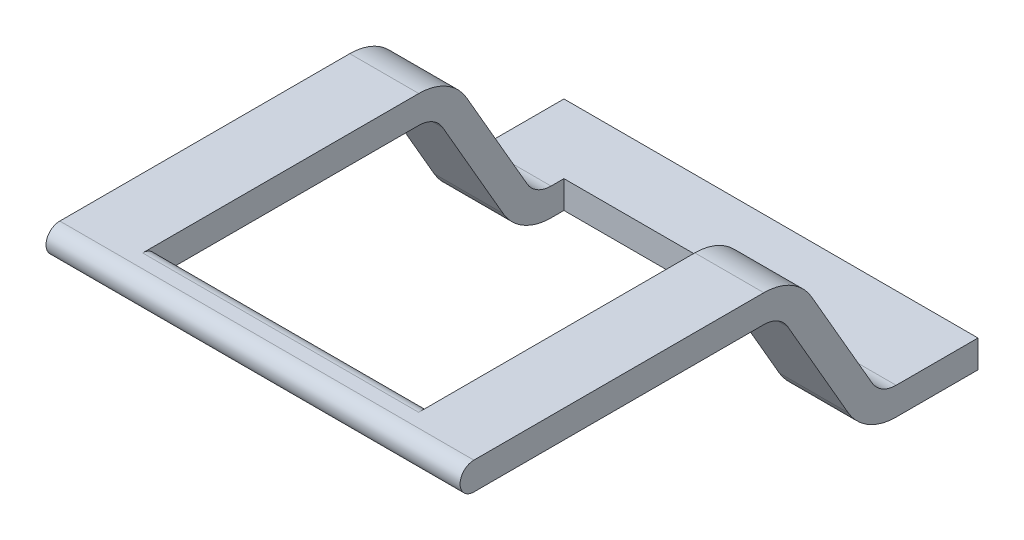
from build123d import *

# Parameters (mm, degrees)
BOSS_EXTRUDE1_DEPTH = 30
CUT_EXTRUDE1_START  = -5
CUT_EXTRUDE1_DEPTH  = 5
BOSS_EXTRUDE2_DEPTH = 1
SKETCH4_W           = 5
SKETCH4_H           = 2
BOSS_EXTRUDE3_DEPTH = 20.16339138
SKETCH5_W           = 5
SKETCH5_H           = 10.599022434
BOSS_EXTRUDE4_DEPTH = 1.154700538
CUT_EXTRUDE2_DEPTH  = 5
BOSS_EXTRUDE5_DEPTH = 1
SKETCH8_W           = 5
SKETCH8_H           = 2
BOSS_EXTRUDE6_DEPTH = 20.16339138
SKETCH9_W           = 5
SKETCH9_H           = 10.599022434
BOSS_EXTRUDE7_DEPTH = 1.154700538
BOSS_EXTRUDE8_DEPTH = 2
DRAFT1_ANGLE        = 30
DRAFT2_ANGLE        = 30
FILLET1_R           = 2
FILLET2_R           = 4


with BuildPart() as part:
    # Sketch1 → Boss-Extrude1 (new body)
    with BuildSketch(Plane(origin=(-30, 0, 0), x_dir=(0, -1, 0), z_dir=(-1, 0, 0))):
        with BuildLine():
            Line((0, -1), (0, -2))
            ThreePointArc((0, -2), (1, -3), (2, -2))
            Line((2, -2), (2, -1))
            ThreePointArc((2, -1), (1, 0), (0, -1))
        make_face()
    extrude(amount=-BOSS_EXTRUDE1_DEPTH)

    # Sketch2 → Cut-Extrude1 (cut)
    with BuildSketch(Plane(origin=(0, 0, 0), x_dir=(0, 0, -1), z_dir=(1, 0, 0)).offset(CUT_EXTRUDE1_START)):
        with BuildLine():
            Line((2, 0), (2, -2))
            ThreePointArc((2, -2), (3, -1), (2, 0))
        make_face()
    extrude(amount=CUT_EXTRUDE1_DEPTH, mode=Mode.SUBTRACT)

    # Sketch3 → Boss-Extrude2 (add)
    with BuildSketch(Plane(origin=(0, 0, -2), x_dir=(-1, 0, 0), z_dir=(0, 0, -1))):
        Polygon((5, -2), (0, -2), (0, 0), (5, 0), (5, -1), align=None)
    extrude(amount=BOSS_EXTRUDE2_DEPTH)

    # Sketch4 → Boss-Extrude3 (add)
    with BuildSketch(Plane(origin=(0, 0, -3), x_dir=(-1, 0, 0), z_dir=(0, 0, -1))):
        with Locations((2.5, -1)):
            Rectangle(SKETCH4_W, SKETCH4_H)
    extrude(amount=BOSS_EXTRUDE3_DEPTH)

    # Sketch5 → Boss-Extrude4 (add)
    with BuildSketch(Plane(origin=(0, 0, -23.16339138), x_dir=(-1, 0, 0), z_dir=(0, 0, -1))):
        with Locations((2.5, -5.299511217)):
            Rectangle(SKETCH5_W, SKETCH5_H)
    extrude(amount=BOSS_EXTRUDE4_DEPTH)

    # Sketch6 → Cut-Extrude2 (cut)
    with BuildSketch(Plane.ZY.offset(30)):
        with BuildLine():
            Line((-2, -2), (-2, 0))
            ThreePointArc((-2, 0), (-3, -1), (-2, -2))
        make_face()
    extrude(amount=-CUT_EXTRUDE2_DEPTH, mode=Mode.SUBTRACT)

    # Sketch7 → Boss-Extrude5 (add)
    with BuildSketch(Plane(origin=(0, 0, -2), x_dir=(-1, 0, 0), z_dir=(0, 0, -1))):
        Polygon((30, -2), (25, -2), (25, -1), (25, 0), (30, 0), align=None)
    extrude(amount=BOSS_EXTRUDE5_DEPTH)

    # Sketch8 → Boss-Extrude6 (add)
    with BuildSketch(Plane(origin=(0, 0, -3), x_dir=(-1, 0, 0), z_dir=(0, 0, -1))):
        with Locations((27.5, -1)):
            Rectangle(SKETCH8_W, SKETCH8_H)
    extrude(amount=BOSS_EXTRUDE6_DEPTH)

    # Sketch9 → Boss-Extrude7 (add)
    with BuildSketch(Plane(origin=(0, 0, -23.16339138), x_dir=(-1, 0, 0), z_dir=(0, 0, -1))):
        with Locations((27.5, -5.299511217)):
            Rectangle(SKETCH9_W, SKETCH9_H)
    extrude(amount=BOSS_EXTRUDE7_DEPTH)

    # Sketch10 → Boss-Extrude8 (add)
    with BuildSketch(Plane.XZ.offset(10.599022434)):
        Polygon((0, -23.16339138), (0, -37.525669468), (-30, -37.525669468), (-30, -23.16339138), (-25, -23.16339138), (-25, -32.525669468), (-5, -32.525669468), (-5, -23.16339138), align=None)
    extrude(amount=BOSS_EXTRUDE8_DEPTH)

    # Draft1
    draft1_faces = [part.faces().sort_by_distance(p)[0] for p in [
        (-2.5, -5.299511217, -24.318091918),
        (-27.5, -5.299511217, -24.318091918),
    ]]
    draft(draft1_faces, Plane(origin=(0, 0, -1), x_dir=(0, 0, 1), z_dir=(0, 1, 0)), DRAFT1_ANGLE)

    # Draft2
    draft2_faces = [part.faces().sort_by_distance(p)[0] for p in [
        (-27.5, -7.299511217, -23.16339138),
        (-2.5, -7.299511217, -23.16339138),
    ]]
    draft(draft2_faces, Plane(origin=(0, -2, -2), x_dir=(0, 0, -1), z_dir=(0, -1, 0)), DRAFT2_ANGLE)

    # Fillet1
    fillet1_edges = [part.edges().sort_by_distance(p)[0] for p in [
        (-27.5, -10.599022434, -30.437440374),
        (-2.5, -2, -23.16339138),
        (-2.5, -10.599022434, -30.437440374),
        (-27.5, -2, -23.16339138),
    ]]
    fillet(fillet1_edges, radius=FILLET1_R)

    # Fillet2
    fillet2_edges = [part.edges().sort_by_distance(p)[0] for p in [
        (-27.5, 0, -24.318091918),
        (-2.5, -12.599022434, -29.282739835),
        (-27.5, -12.599022434, -29.282739835),
        (-2.5, 0, -24.318091918),
    ]]
    fillet(fillet2_edges, radius=FILLET2_R)


solid = part.part
